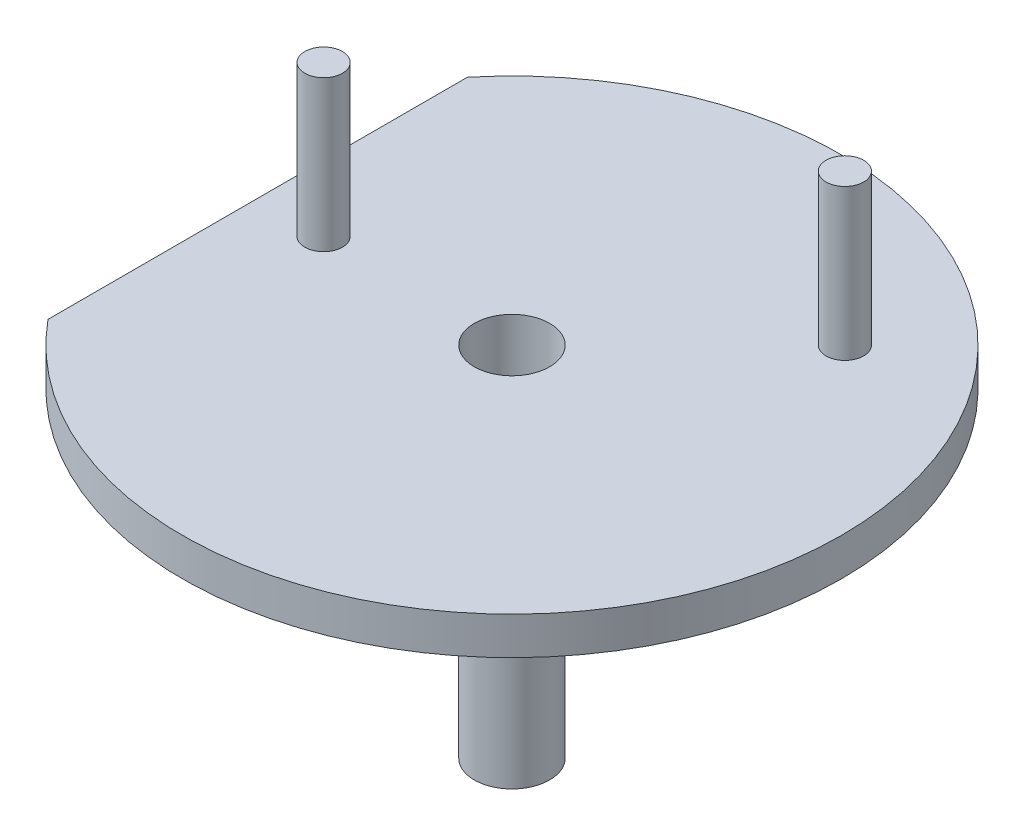
from build123d import *

# Parameters (mm, degrees)
SKETCH1_R           = 17.5
BOSS_EXTRUDE1_DEPTH = 2
SKETCH3_R           = 4
BOSS_EXTRUDE2_DEPTH = 2
CHAMFER1_SIZE       = 1
SKETCH4_R           = 2
BOSS_EXTRUDE3_DEPTH = 15
SKETCH5_R           = 1.5
CUT_EXTRUDE1_DEPTH  = 15
SKETCH6_R           = 1
BOSS_EXTRUDE4_DEPTH = 8
SKETCH7_W           = 4
SKETCH7_H           = 45.60719986
CUT_EXTRUDE2_DEPTH  = 32.200961524
SKETCH8_R           = 2
CUT_EXTRUDE3_DEPTH  = 3


with BuildPart() as part:
    # Sketch1 → Boss-Extrude1 (new body)
    with BuildSketch(Plane(origin=(0, 0, 0), x_dir=(1, 0, 0), z_dir=(0, 1, 0))):
        with Locations(Location((0, 0, 0), (0, 0, 270))):
            Circle(SKETCH1_R)
    extrude(amount=BOSS_EXTRUDE1_DEPTH)

    # Sketch3 → Boss-Extrude2 (add)
    with BuildSketch(Plane.XZ):
        with Locations(Location((0, 0, 0), (0, 0, 270))):
            Circle(SKETCH3_R)
    extrude(amount=BOSS_EXTRUDE2_DEPTH)

    # Chamfer1
    chamfer1_edges = [part.edges().sort_by_distance(p)[0] for p in [
        (0, 0, 4),
    ]]
    chamfer(chamfer1_edges, length=CHAMFER1_SIZE)

    # Sketch4 → Boss-Extrude3 (add)
    with BuildSketch(Plane.XZ.offset(2)):
        with Locations(Location((0, 0, 0), (0, 0, 270))):
            Circle(SKETCH4_R)
    extrude(amount=BOSS_EXTRUDE3_DEPTH)

    # Sketch5 → Cut-Extrude1 (cut)
    with BuildSketch(Plane.XZ.offset(17)):
        with Locations(Location((0, 0, 0), (0, 0, 270))):
            Circle(SKETCH5_R)
    extrude(amount=-CUT_EXTRUDE1_DEPTH, mode=Mode.SUBTRACT)

    # Sketch6 → Boss-Extrude4 (add)
    with BuildSketch(Plane(origin=(0, 2, 0), x_dir=(1, 0, 0), z_dir=(0, 1, 0))):
        with Locations(Location((-10, 0, 0), (0, 0, 270))):
            Circle(SKETCH6_R)
        with Locations(Location((8.838834765, 8.838834765, 0), (0, 0, 270))):
            Circle(SKETCH6_R)
    extrude(amount=BOSS_EXTRUDE4_DEPTH)

    # Sketch7 → Cut-Extrude2 (cut, through all)
    with BuildSketch(Plane(origin=(0, 2, 0), x_dir=(1, 0, 0), z_dir=(0, 1, 0))):
        with Locations((-15.5, 0)):
            Rectangle(SKETCH7_W, SKETCH7_H)
    extrude(amount=-CUT_EXTRUDE2_DEPTH, mode=Mode.SUBTRACT)

    # Sketch8 → Cut-Extrude3 (cut)
    with BuildSketch(Plane(origin=(0, 2, 0), x_dir=(1, 0, 0), z_dir=(0, 1, 0))):
        with Locations(Location((0, 0, 0), (0, 0, 90))):
            Circle(SKETCH8_R)
    extrude(amount=-CUT_EXTRUDE3_DEPTH, mode=Mode.SUBTRACT)


solid = part.part
